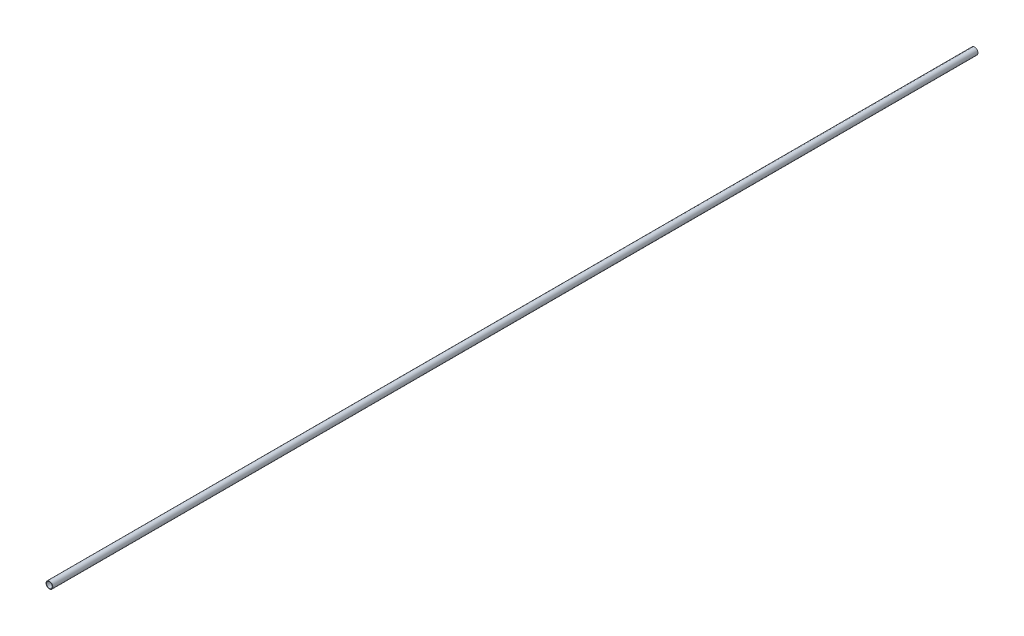
from build123d import *

# Parameters (mm, degrees)
SKETCH_1_R      = 12.5
SKETCH_1_R_2    = 10.5
EXTRUDE_1_DEPTH = 1700


with BuildPart() as part:
    # 草图1 → 凸台-拉伸1 (new, symmetric)
    with BuildSketch(Plane.XY):
        Circle(SKETCH_1_R)
        Circle(SKETCH_1_R_2, mode=Mode.SUBTRACT)
    extrude(amount=EXTRUDE_1_DEPTH, both=True)


solid = part.part
